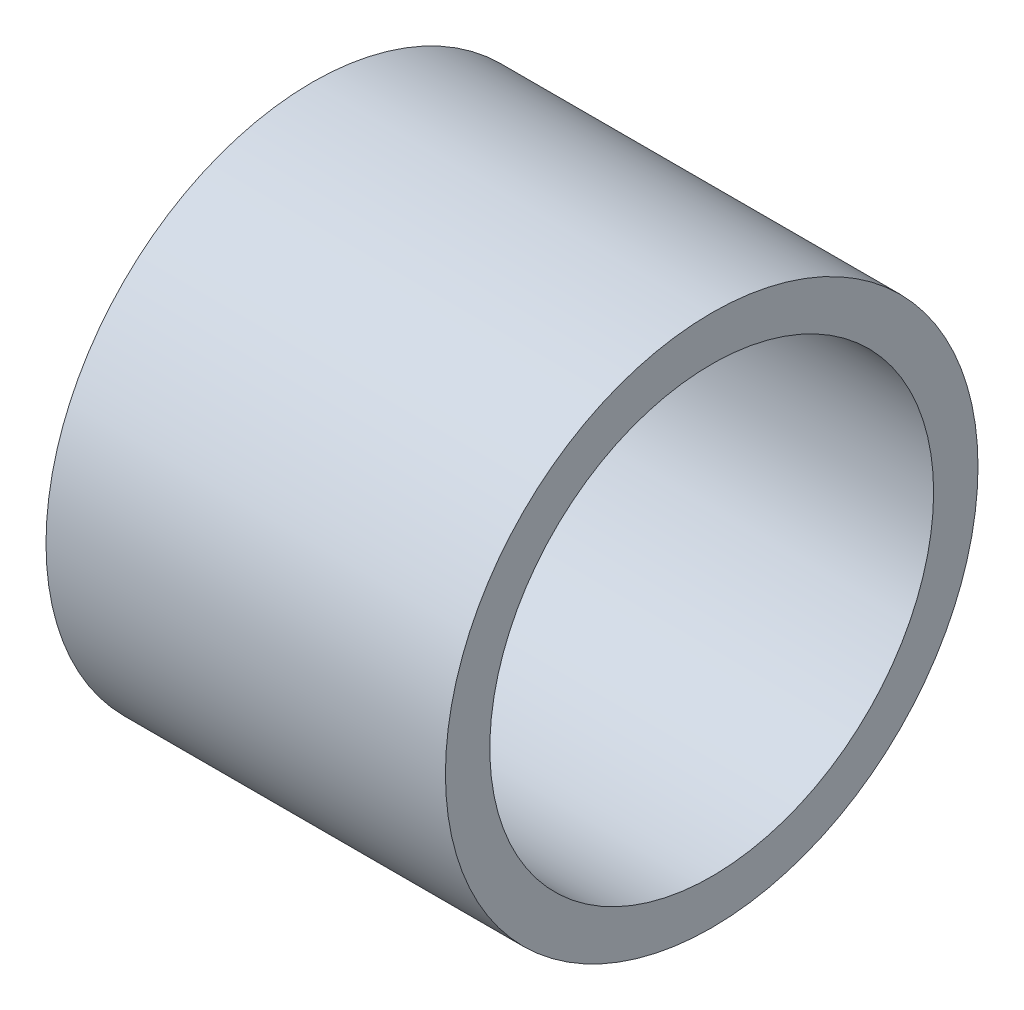
SolidWorks part; units mm, degrees
ref_plane "Front" through (0, 0, 0) normal (0, 0, 1) x (1, 0, 0)
ref_plane "Top" through (0, 0, 0) normal (0, 1, 0) x (1, 0, 0)
ref_plane "Right" through (0, 0, 0) normal (1, 0, 0) x (0, 0, -1)
sketch "Sketch1" plane through (0, 0, 0) normal (1, 0, 0) x (0, 0, -1)
  circle A0 centre (0, 0) radius 10
  circle A1 centre (0, 0) radius 12
  dimension "D1" = 20
  dimension "D2" = 24
extrude "Boss-Extrude1" add sketch "Sketch1" along normal blind 18
